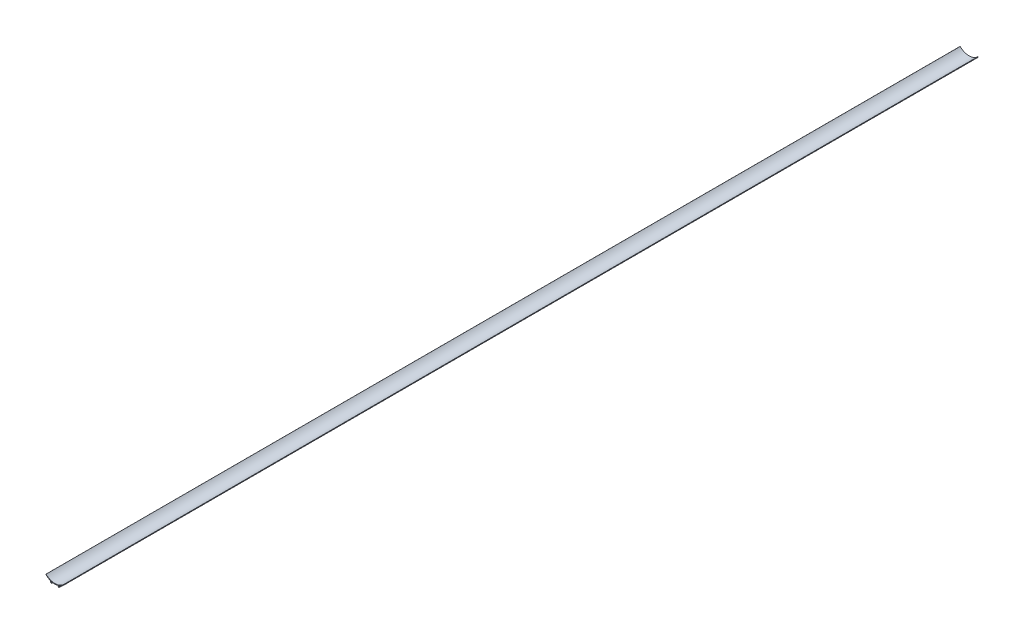
from build123d import *

# Parameters (mm, degrees)
EXTRUDE_1_DEPTH = 1195


with BuildPart() as part:
    # 草图2 → 凸台-拉伸1 (new, symmetric)
    with BuildSketch(Plane.XY):
        with BuildLine():
            Line((-11.25, 5.782842712), (-10.667157288, 5.199999999))
            Line((-10.667157288, 5.199999999), (-8.25, 5.199999999))
            Line((-8.25, 5.199999999), (-8.25, 6))
            Line((-8.25, 6), (-10.25, 6))
            Line((-10.25, 6), (-10.25, 7.726142057))
            Line((-10.25, 7.726142057), (-8.999999375, 7.724528349))
            Line((-8.999999375, 7.724528349), (-8.25, 8.473560125))
            Line((-8.25, 8.473560125), (-8.25, 8.88650173))
            ThreePointArc((-8.25, 8.88650173), (-5.642322013, 8.341793831), (-3, 8.002934636))
            Line((-3, 8.002934636), (-3, 7.70225919))
            Line((-3, 7.70225919), (3, 7.70225919))
            Line((3, 7.70225919), (3, 8.002934636))
            ThreePointArc((3, 8.002934636), (5.642322013, 8.341793831), (8.25, 8.88650173))
            Line((8.25, 8.88650173), (8.25, 8.473560125))
            Line((8.25, 8.473560125), (8.999999375, 7.724528349))
            Line((8.999999375, 7.724528349), (10.25, 7.726142057))
            Line((10.25, 7.726142057), (10.25, 6))
            Line((10.25, 6), (8.25, 6))
            Line((8.25, 6), (8.25, 5.2))
            Line((8.25, 5.2), (10.667157288, 5.2))
            Line((10.667157288, 5.2), (11.25, 5.782842712))
            Line((11.25, 5.782842712), (11.25, 9.785632758))
            ThreePointArc((11.25, 9.785632758), (17.712457567, 12.84892987), (23.391097866, 17.196364903))
            Line((23.391097866, 17.196364903), (23.391097866, 18.63499481))
            ThreePointArc((23.391097866, 18.63499481), (23.329308001, 18.727406852), (23.220298155, 18.705616343))
            ThreePointArc((23.220298155, 18.705616343), (0, 9.070311977), (-23.220298155, 18.705616342))
            ThreePointArc((-23.220298155, 18.705616342), (-23.329308002, 18.727406852), (-23.391097866, 18.634994809))
            Line((-23.391097866, 18.634994809), (-23.391097866, 17.196364902))
            ThreePointArc((-23.391097866, 17.196364902), (-17.712457568, 12.84892987), (-11.25, 9.785632758))
            Line((-11.25, 9.785632758), (-11.25, 5.782842712))
        make_face()
    extrude(amount=EXTRUDE_1_DEPTH, both=True)


solid = part.part
